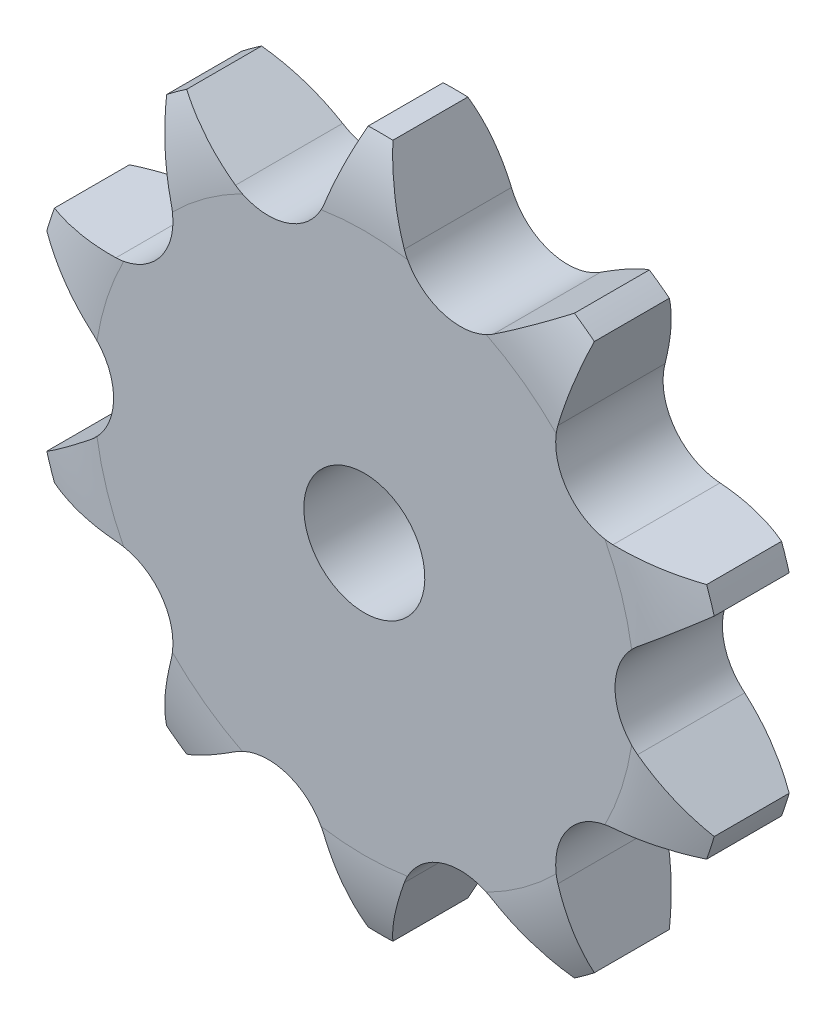
from build123d import *

# Parameters (mm, degrees)
CUT_EXTRUDE_1_DEPTH      = 74.277691012
PATTERN_CIRCULAR_1_COUNT = 10


with BuildPart() as part:
    # 草图4 → 旋转1 (revolve)
    with BuildSketch(Plane(origin=(0, 0, 0), x_dir=(0, 0, -1), z_dir=(1, 0, 0))):
        with BuildLine():
            Line((-19.8, 35.775702269), (-19.8, 8))
            Line((-19.8, 8), (-34, 8))
            Line((-34, 8), (-34, 35.775702269))
            ThreePointArc((-34, 35.775702269), (-33.458696863, 40.949883148), (-31.858228179, 45.9))
            Line((-31.858228179, 45.9), (-21.941771821, 45.9))
            ThreePointArc((-21.941771821, 45.9), (-20.341303137, 40.949883148), (-19.8, 35.775702269))
        make_face()
    revolve(axis=Axis((0, 0, 0), (0, 0, 1)))

    # 草图5 → 切除-拉伸1 (cut, through all)
    with BuildSketch(Plane.XY):
        with BuildLine():
            Line((1.25, 46.883339258), (5.275977282, 36.26778067))
            ThreePointArc((5.275977282, 36.26778067), (10.246222168, 31.53203064), (17.05088284, 32.44156663))
            Line((17.05088284, 32.44156663), (26.547937038, 38.662863823))
            ThreePointArc((26.547937038, 38.662863823), (14.49397737, 44.604199578), (1.25, 46.883339258))
        make_face()
    cut_extrude_1 = extrude(amount=CUT_EXTRUDE_1_DEPTH, mode=Mode.SUBTRACT)

    # 阵列(圆周)1: 切除-拉伸1 ×10 about axis
    pattern_circular_1_axis = Axis((0, 0, 0), (0, 0, 1))
    for i in range(1, PATTERN_CIRCULAR_1_COUNT):
        add(cut_extrude_1.rotate(pattern_circular_1_axis, i * 360 / PATTERN_CIRCULAR_1_COUNT), mode=Mode.SUBTRACT)


solid = part.part
